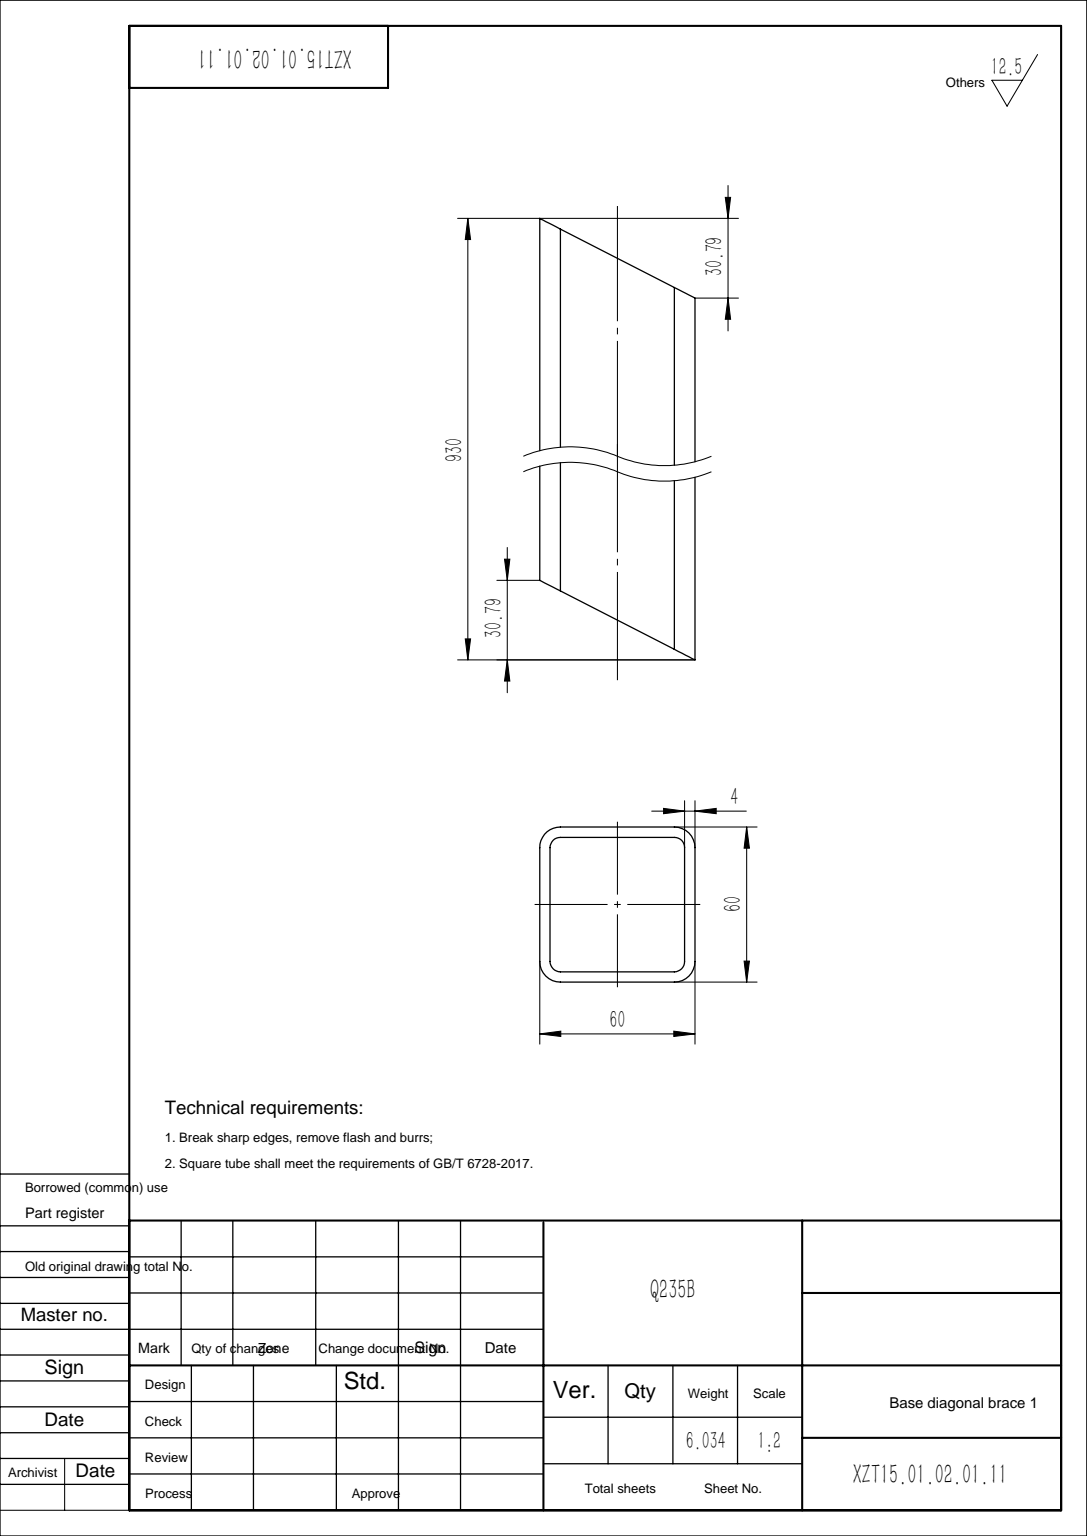
SolidWorks part; units mm, degrees
material "Q235B"
ref_plane "Front Plane" through (0, 0, 0) normal (0, 0, 1) x (1, 0, 0)
ref_plane "Top Plane" through (0, 0, 0) normal (0, 1, 0) x (1, 0, 0)
ref_plane "Right Plane" through (0, 0, 0) normal (1, 0, 0) x (0, 0, -1)
sketch "草图1" plane through (0, 0, 0) normal (0, 0, 1) x (1, 0, 0)
  line L0 (0, 0) -> (0, 930)
  dimension "D1" = 930
other "GB/T 6728-2002 square hollow section 60×60×4(1)"
ref_plane "Plane1" through (0, 0, 0) normal (0, 1, 0) x (-1, 0, 0)
sketch "Sketch1" plane through (0, 0, 0) normal (0, 1, 0) x (-1, 0, 0)
  line L0 (-22, -26) -> (22, -26)
  line L1 (-26, -22) -> (-26, 22)
  line L2 (22, 26) -> (-22, 26)
  line L3 (26, 22) -> (26, -22)
  line L4 (-22, -30) -> (22, -30)
  line L5 (-30, -22) -> (-30, 22)
  line L6 (22, 30) -> (-22, 30)
  line L7 (30, 22) -> (30, -22)
  arc A0 (30, 22) -> (22, 30) centre (22, 22) ccw
  arc A1 (22, -30) -> (30, -22) centre (22, -22) ccw
  arc A2 (-30, -22) -> (-22, -30) centre (-22, -22) ccw
  arc A3 (-22, 30) -> (-30, 22) centre (-22, 22) ccw
  arc A4 (-22, 26) -> (-26, 22) centre (-22, 22) ccw
  arc A5 (26, 22) -> (22, 26) centre (22, 22) ccw
  arc A6 (22, -26) -> (26, -22) centre (22, -22) ccw
  arc A7 (-26, -22) -> (-22, -26) centre (-22, -22) ccw
  point P0 (-30, 0)
  point P1 (30, 0)
  point P2 (0, 30)
  point P3 (0, -30)
  point P4 (0, 0)
  point P5 (-30, -30)
  point P6 (30, -30)
  point P7 (30, 30)
  point P8 (-30, 30)
  point P33 (0, 0)
  dimension "D1" = 8
  dimension "Thickness" = 4
  dimension "V_leg" = 60
sketch "Sketch2" plane through (0, 0, 30) normal (0, 0, 1) x (1, 0, 0)
  line L0 (-30, 930) -> (30, 899.2068)
  line L1 (30, 930) -> (30, 0) construction
  line L2 (30, 899.2068) -> (30, 930)
  line L3 (30, 930) -> (-30, 930)
  line L4 (-30, 0) -> (-30, 30.7932)
  line L5 (-30, 930) -> (-30, 0) construction
  line L6 (-30, 30.7932) -> (30, 0)
  line L7 (30, 0) -> (-30, 0)
  dimension "D1" = 800
  dimension "D2" = 30.7932
extrude "Cut-Extrude1" cut sketch "Sketch2" against normal through all both and the other way through all
